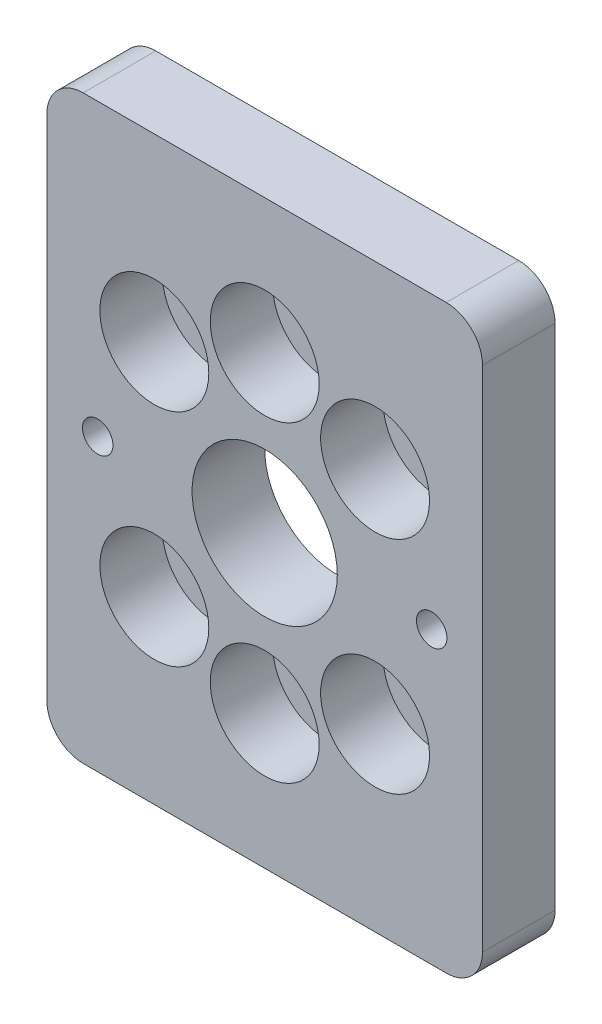
from build123d import *

# Parameters (mm, degrees)
SKETCH1_W                                           = 60
SKETCH1_H                                           = 80
SKETCH1_R                                           = 10
SKETCH1_R_2                                         = 2
BOSS_EXTRUDE1_DEPTH                                 = 10
M5_TAPPED_HOLE1_D                                   = 4.2
CBORE_FOR_M8_HEX_SOCKET_HEAD_CAP_SCREW1_D           = 9
CBORE_FOR_M8_HEX_SOCKET_HEAD_CAP_SCREW1_CBORE_D     = 15
CBORE_FOR_M8_HEX_SOCKET_HEAD_CAP_SCREW1_CBORE_DEPTH = 8.6
CIRPATTERN1_COUNT                                   = 8
FILLET1_R                                           = 5


with BuildPart() as part:
    # Sketch1 → Boss-Extrude1 (new body)
    with BuildSketch(Plane.XY):
        Rectangle(SKETCH1_W, SKETCH1_H)
        Circle(SKETCH1_R, mode=Mode.SUBTRACT)
        with Locations((-23, 0)):
            Circle(SKETCH1_R_2, mode=Mode.SUBTRACT)
        with Locations(Location((23, 0, 0), (0, 0, 180))):
            Circle(SKETCH1_R_2, mode=Mode.SUBTRACT)
    extrude(amount=BOSS_EXTRUDE1_DEPTH)

    # M5 Tapped Hole1 (through all)
    with Locations(Plane.XY.offset(10)):
        with Locations((-23, 0), (23, 0)):
            Hole(M5_TAPPED_HOLE1_D / 2)

    # CBORE for M8 Hex Socket Head Cap Screw1 (through all)
    with Locations(Plane.XY.offset(10)):
        with Locations((0, 21.5)):
            cbore_for_m8_hex_socket_head_cap_screw1 = CounterBoreHole(CBORE_FOR_M8_HEX_SOCKET_HEAD_CAP_SCREW1_D / 2, CBORE_FOR_M8_HEX_SOCKET_HEAD_CAP_SCREW1_CBORE_D / 2, CBORE_FOR_M8_HEX_SOCKET_HEAD_CAP_SCREW1_CBORE_DEPTH)

    # CirPattern1: CBORE for M8 Hex Socket Head Cap Screw1 ×8 about axis, 2 skipped
    cirpattern1_axis = Axis((0, 0, 0), (0, 0, 1))
    add([cbore_for_m8_hex_socket_head_cap_screw1.rotate(cirpattern1_axis, i * 360 / CIRPATTERN1_COUNT) for i in range(1, CIRPATTERN1_COUNT) if i not in (2, 6)], mode=Mode.SUBTRACT)

    # Fillet1
    fillet1_edges = [part.edges().sort_by_distance(p)[0] for p in [
        (30, -40, 5),
        (-30, -40, 5),
        (-30, 40, 5),
        (30, 40, 5),
    ]]
    fillet(fillet1_edges, radius=FILLET1_R)


solid = part.part
